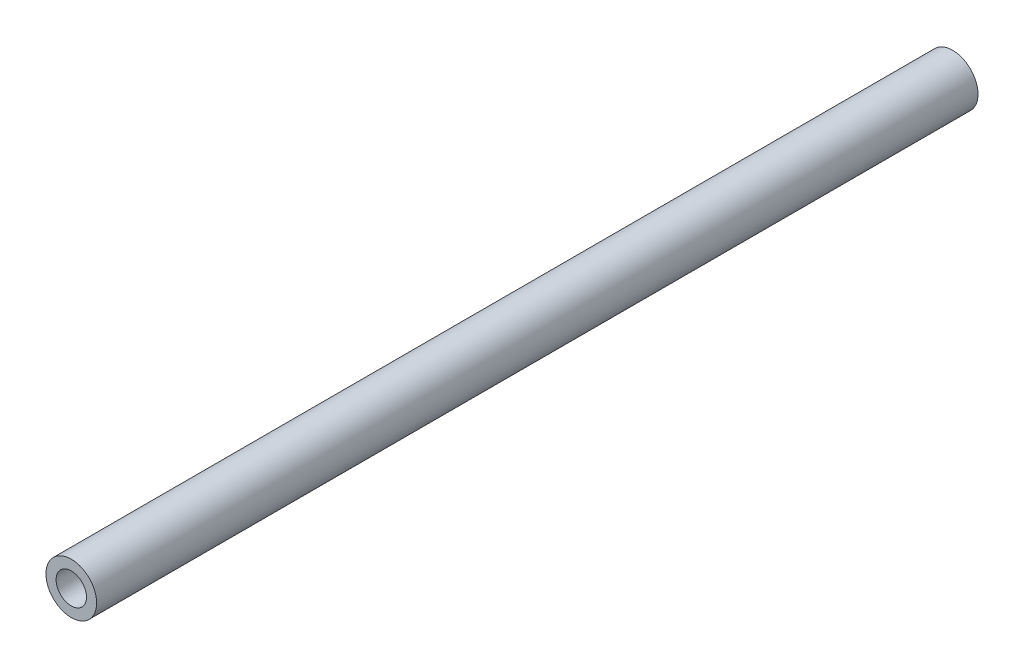
SolidWorks part; units mm, degrees
ref_plane "Front Plane" through (0, 0, 0) normal (0, 0, 1) x (1, 0, 0)
ref_plane "Top Plane" through (0, 0, 0) normal (0, 1, 0) x (1, 0, 0)
ref_plane "Right Plane" through (0, 0, 0) normal (1, 0, 0) x (0, 0, -1)
sketch "Sketch1" plane through (0, 0, 0) normal (0, 0, 1) x (1, 0, 0)
  circle A0 centre (0, 0) radius 5
  dimension "D1" = 10
extrude "Boss-Extrude1" add sketch "Sketch1" along normal mid plane 174
sketch "Sketch2" plane through (0, 0, 87) normal (0, 0, 1) x (1, 0, 0)
  circle A0 centre (0, 0) radius 3
  dimension "D1" = 6
extrude "Cut-Extrude1" cut sketch "Sketch2" against normal blind 10
mirror "Mirror1" about plane through (0, 0, 0) normal (0, 0, 1) of "Cut-Extrude1"
